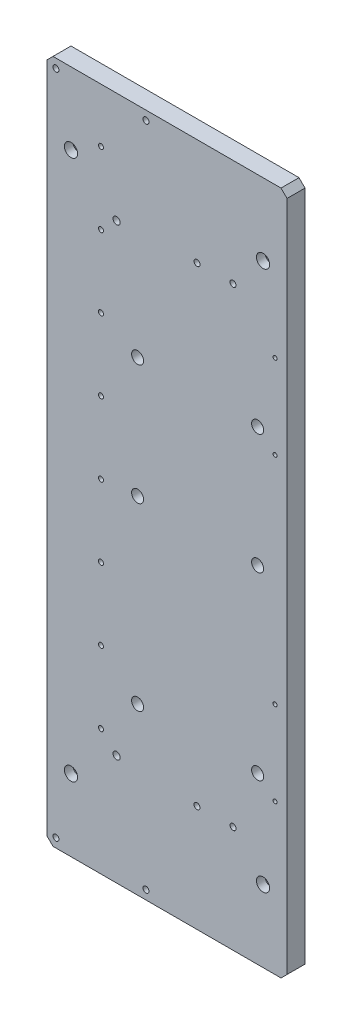
SolidWorks part; units mm, degrees
material "6061"
ref_plane "前视基准面" through (0, 0, 0) normal (0, 0, 1) x (1, 0, 0)
ref_plane "上视基准面" through (0, 0, 0) normal (0, 1, 0) x (1, 0, 0)
ref_plane "右视基准面" through (0, 0, 0) normal (1, 0, 0) x (0, 0, -1)
sketch "草图1" plane through (0, 0, 0) normal (0, 0, 1) x (1, 0, 0)
  line L1 (-100, -285) -> (100, -285)
  line L2 (-100, -285) -> (-100, 285)
  line L3 (-100, 285) -> (100, 285)
  line L4 (100, -285) -> (100, 285)
  line L5 (-100, -285) -> (100, 285) construction
  line L6 (-100, 285) -> (100, -285) construction
  point P0 (0, 0)
  dimension "D1" = 570
  dimension "D2" = 200
extrude "凸台-拉伸1" add sketch "草图1" along normal blind 15
chamfer "倒角1" distance 5 angle 45 4 edges at (100, 285, 7.5) (-100, 285, 7.5) (-100, -285, 7.5) (100, -285, 7.5)
hole_wizard "大小mm 暗销孔0" positions "草图6" profile "草图7" hole size "Ø6.0" standard "ISO" end condition through all
sketch "草图6" plane through (0, 0, 15) normal (0, 0, 1) x (1, 0, 0)
  line L0 (-100, -193) -> (345.8941, -193) construction
  line L1 (-100, 280) -> (-100, -280) construction
  line L3 (-95, -285) -> (95, -285) construction
  line L4 (-100, 0) -> (345.8941, 0) construction
  point P0 (-42, -193)
  point P2 (258, -193)
  point P13 (-100, 0)
  point P14 (-42, 193)
  point P16 (258, 193)
  dimension "D1" = 92
  dimension "D2" = 58
  dimension "D3" = 300
sketch "草图7" plane through (-42, -193, 15) normal (1, 0, 0) x (0, -1, 0)
  line L0 (0, 0) -> (0, 15)
  line L1 (0, 15) -> (3, 15)
  line L2 (3, 15) -> (3, 0)
  line L5 (3, 0) -> (0, 0)
  line L11 (0, -6.35) -> (0, 107.95) construction
  dimension "通孔孔直径" = 6
  dimension "通孔孔深度" = 15
hole_wizard "M6 螺纹孔1" positions "草图8" profile "草图9" tap size "M6" standard "ISO" end condition through all
sketch "草图8" plane through (0, 0, 15) normal (0, 0, 1) x (1, 0, 0)
  point P0 (55, 196)
  point P3 (25, 196)
  point P6 (55, -196)
  point P9 (25, -196)
sketch "草图9" plane through (55, 196, 15) normal (1, 0, 0) x (0, -1, 0)
  line L0 (0, 0) -> (0, 15)
  line L1 (0, 15) -> (2.5, 15)
  line L2 (2.5, 15) -> (2.5, 0)
  line L5 (2.5, 0) -> (0, 0)
  line L11 (0, -6.35) -> (0, 107.95) construction
  dimension "通孔螺纹孔钻头直径" = 5
  dimension "通孔螺纹孔钻头深度" = 15
cosmetic thread "孔螺蚊线1" parameters "D2"=6
cosmetic thread "孔螺蚊线2" parameters "D2"=6
cosmetic thread "孔螺蚊线3" parameters "D2"=6
cosmetic thread "孔螺蚊线4" parameters "D2"=6
hole_wizard "M5 螺纹孔2" positions "草图10" profile "草图11" tap size "M5" standard "ISO" end condition through all
sketch "草图10" plane through (0, 0, 15) normal (0, 0, 1) x (1, 0, 0)
  point P0 (-55, 240)
  point P3 (-55, 180)
  point P6 (-55, 120)
  point P9 (-55, 60)
  point P12 (-55, 0)
  point P15 (-55, -60)
  point P18 (-55, -120)
  point P21 (-55, -180)
sketch "草图11" plane through (-55, 240, 15) normal (1, 0, 0) x (0, -1, 0)
  line L0 (0, 0) -> (0, 15)
  line L1 (0, 15) -> (2.1, 15)
  line L2 (2.1, 15) -> (2.1, 0)
  line L5 (2.1, 0) -> (0, 0)
  line L11 (0, -6.35) -> (0, 107.95) construction
  dimension "通孔螺纹孔钻头直径" = 4.2
  dimension "通孔螺纹孔钻头深度" = 15
cosmetic thread "孔螺蚊线5" parameters "D2"=5
cosmetic thread "孔螺蚊线6" parameters "D2"=5
cosmetic thread "孔螺蚊线7" parameters "D2"=5
cosmetic thread "孔螺蚊线8" parameters "D2"=5
cosmetic thread "孔螺蚊线9" parameters "D2"=5
cosmetic thread "孔螺蚊线10" parameters "D2"=5
cosmetic thread "孔螺蚊线11" parameters "D2"=5
cosmetic thread "孔螺蚊线12" parameters "D2"=5
hole_wizard "M6 螺纹孔2" positions "草图12" profile "草图13" tap size "M6" standard "GB" end condition through all
sketch "草图12" plane through (0, 0, 15) normal (0, 0, 1) x (1, 0, 0)
  point P0 (-92.5, -277.5)
  point P3 (-17.5, -277.5)
  point P7 (-17.5, 277.5)
  point P10 (-92.5, 277.5)
sketch "草图13" plane through (-92.5, -277.5, 15) normal (1, 0, 0) x (0, -1, 0)
  line L0 (0, 0) -> (0, 15)
  line L1 (0, 15) -> (2.5, 15)
  line L2 (2.5, 15) -> (2.5, 0)
  line L5 (2.5, 0) -> (0, 0)
  line L11 (0, -6.35) -> (0, 107.95) construction
  dimension "通孔螺纹孔钻头直径" = 5
  dimension "通孔螺纹孔钻头深度" = 15
cosmetic thread "孔螺蚊线14" parameters "D2"=6
cosmetic thread "孔螺蚊线15" parameters "D2"=6
cosmetic thread "孔螺蚊线21" parameters "D2"=6
cosmetic thread "孔螺蚊线22" parameters "D2"=6
hole_wizard "M4 螺纹孔1" positions "草图14" profile "草图15" tap size "M4" standard "GB" end condition through all
sketch "草图14" plane through (0, 0, 15) normal (0, 0, 1) x (1, 0, 0)
  line L0 (90, -172.25) -> (90, -147.75) construction
  line L2 (90, -102.25) -> (90, -77.75) construction
  line L4 (90, 77.75) -> (90, 102.25) construction
  line L6 (90, 147.75) -> (90, 172.25) construction
  arc A0 (87.75, -170) -> (92.25, -170) centre (90, -170) ccw construction
  arc A1 (92.25, -150) -> (87.75, -150) centre (90, -150) ccw construction
  arc A2 (87.75, -100) -> (92.25, -100) centre (90, -100) ccw construction
  arc A3 (92.25, -80) -> (87.75, -80) centre (90, -80) ccw construction
  arc A4 (87.75, 80) -> (92.25, 80) centre (90, 80) ccw construction
  arc A5 (92.25, 100) -> (87.75, 100) centre (90, 100) ccw construction
  arc A6 (87.75, 150) -> (92.25, 150) centre (90, 150) ccw construction
  arc A7 (92.25, 170) -> (87.75, 170) centre (90, 170) ccw construction
  point P0 (90, -160)
  point P42 (90, -90)
  point P44 (90, 90)
  point P46 (90, 160)
sketch "草图15" plane through (90, -160, 15) normal (1, 0, 0) x (0, -1, 0)
  line L0 (0, 0) -> (0, 15)
  line L1 (0, 15) -> (1.65, 15)
  line L2 (1.65, 15) -> (1.65, 0)
  line L5 (1.65, 0) -> (0, 0)
  line L11 (0, -6.35) -> (0, 107.95) construction
  dimension "通孔螺纹孔钻头直径" = 3.3
  dimension "通孔螺纹孔钻头深度" = 15
cosmetic thread "孔螺蚊线17" parameters "D2"=4
cosmetic thread "孔螺蚊线18" parameters "D2"=4
cosmetic thread "孔螺蚊线19" parameters "D2"=4
cosmetic thread "孔螺蚊线20" parameters "D2"=4
hole_wizard "大小mm 暗销孔1" positions "草图16" profile "草图17" hole size "Ø1.0" standard "ISO"
sketch "草图16" plane through (0, 0, 0) normal (0, 0, -1) x (-1, 0, 0)
  point P0 (24.5, 103)
  point P3 (-75.5, 103)
  point P6 (24.5, -147)
  point P9 (-75.5, -147)
  point P12 (24.5, 3)
  point P15 (-75.5, 3)
sketch "草图17" plane through (-24.5, 103, 0) normal (1, 0, 0) x (0, 1, 0)
  line L0 (0, 0) -> (0, 17.3004)
  line L1 (0, 17.3004) -> (0.5, 17)
  line L2 (0.5, 17) -> (0.5, 0)
  line L5 (0.5, 0) -> (0, 0)
  line L10 (0, 17.3004) -> (-0.5, 17) construction
  line L11 (0, -6.35) -> (0, 107.95) construction
  dimension "孔直径" = 1
  dimension "孔深度" = 17
  dimension "导头角度" = 118
hole_wizard "M5 六角凹头螺钉的柱形沉头孔1" positions "草图18" profile "草图19" counterbore size "M5" standard "ISO"
sketch "草图18" plane through (0, 0, 15) normal (0, 0, 1) x (1, 0, 0)
  point P0 (75.5, -147)
  point P3 (75.5, 103)
  point P6 (75.5, 3)
  point P9 (-24.5, 103)
  point P12 (-24.5, 3)
  point P15 (-24.5, -147)
sketch "草图19" plane through (75.5, -147, 15) normal (1, 0, 0) x (0, -1, 0)
  line L0 (0, 0) -> (0, 18.6524)
  line L1 (0, 18.6524) -> (2.75, 17)
  line L2 (2.75, 17) -> (2.75, 7)
  line L3 (2.75, 7) -> (5, 7)
  line L4 (5, 7) -> (5, 0)
  line L5 (5, 0) -> (0, 0)
  line L10 (0, 18.6524) -> (-2.75, 17) construction
  line L11 (0, -6.35) -> (0, 107.95) construction
  dimension "孔直径" = 5.5
  dimension "孔深度" = 17
  dimension "柱形沉头孔直径" = 10
  dimension "柱形沉头孔深度" = 7
  dimension "导头角度" = 118
hole_wizard "打孔尺寸(%根据)内六角花形圆柱头螺钉1" positions "草图22" profile "草图23" counterbore size "M6" standard "GB" end condition through all
sketch "草图22" plane through (0, 0, 15) normal (0, 0, 1) x (1, 0, 0)
  line L1 (-80, -225) -> (80, -225)
  line L2 (-80, -225) -> (-80, 225)
  line L3 (-80, 225) -> (80, 225)
  line L4 (80, -225) -> (80, 225)
  line L5 (-80, -225) -> (80, 225)
  point P0 (-80, -225)
  point P2 (80, -225)
  point P4 (-80, 225)
  point P6 (80, 225)
  dimension "D1" = 160
  dimension "D2" = 450
sketch "草图23" plane through (-80, -225, 15) normal (1, 0, 0) x (0, -1, 0)
  line L0 (0, 0) -> (0, 15)
  line L1 (0, 15) -> (3.3, 15)
  line L3 (3.3, 15) -> (3.3, 7)
  line L4 (3.3, 7) -> (5.5, 7)
  line L5 (5.5, 7) -> (5.5, 0)
  line L7 (5.5, 0) -> (0, 0)
  line L11 (0, -6.35) -> (0, 107.95) construction
  dimension "通孔孔直径" = 6.6
  dimension "通孔孔深度" = 15
  dimension "柱形沉头孔直径" = 11
  dimension "柱形沉头孔深度" = 7
